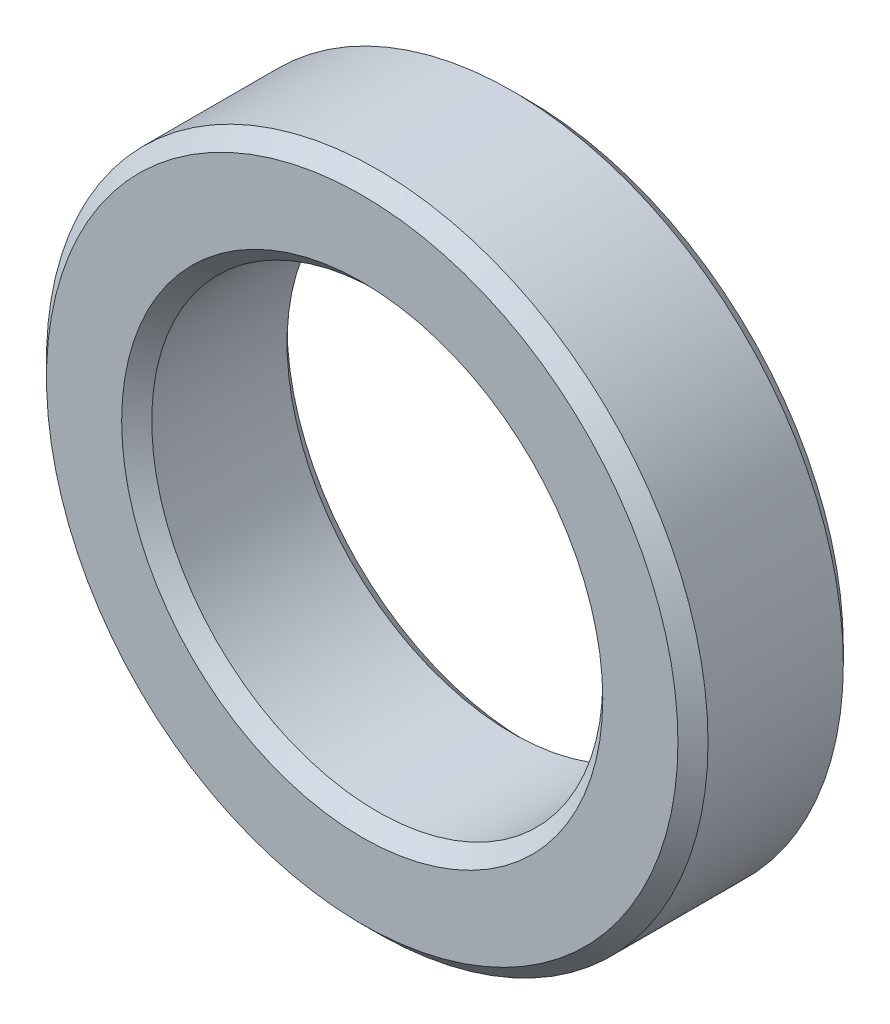
from build123d import *

# Parameters (mm, degrees)
SKETCH1_R           = 11
SKETCH1_R_2         = 7.5
BOSS_EXTRUDE1_DEPTH = 5.5
CHAMFER1_SIZE       = 0.5


with BuildPart() as part:
    # Sketch1 → Boss-Extrude1 (new body)
    with BuildSketch(Plane.XY):
        Circle(SKETCH1_R)
        Circle(SKETCH1_R_2, mode=Mode.SUBTRACT)
    extrude(amount=BOSS_EXTRUDE1_DEPTH)

    # Chamfer1
    chamfer1_edges = [part.edges().sort_by_distance(p)[0] for p in [
        (-11, 0, 0),
        (-11, 0, 5.5),
        (-7.5, 0, 0),
        (-7.5, 0, 5.5),
    ]]
    chamfer(chamfer1_edges, length=CHAMFER1_SIZE)


solid = part.part
